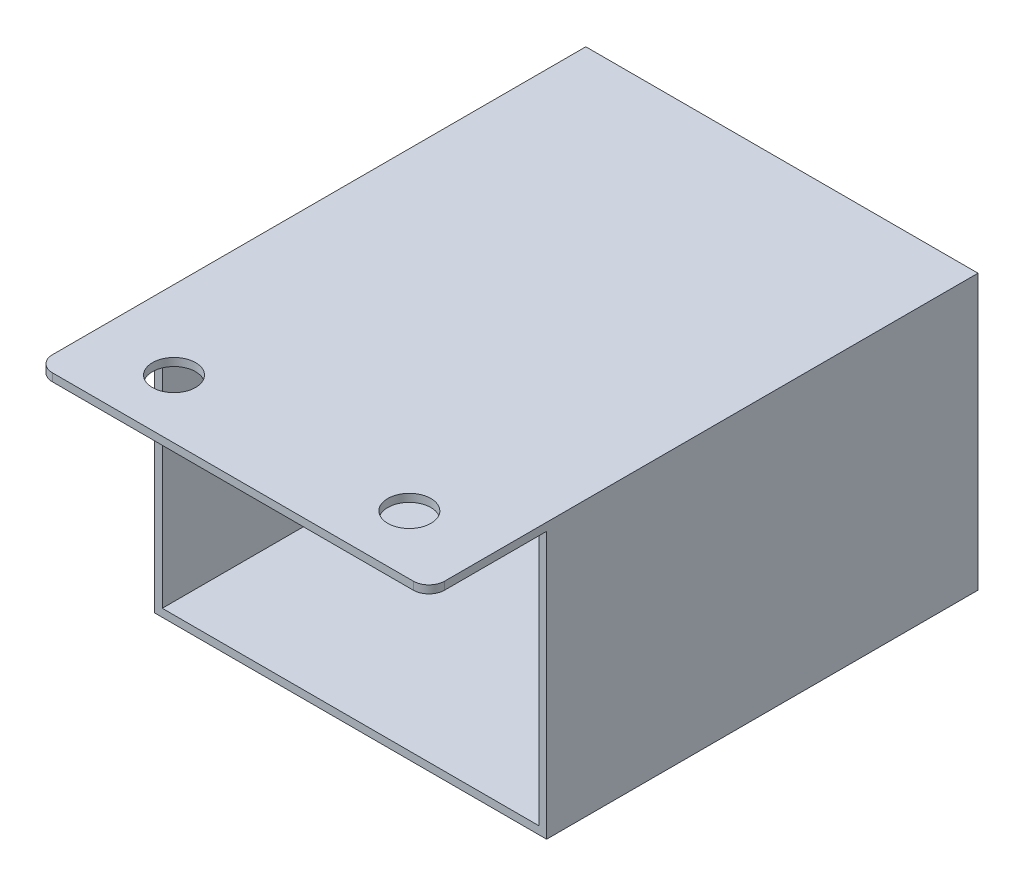
SolidWorks part; units mm, degrees
ref_plane "前视基准面" through (0, 0, 0) normal (0, 0, 1) x (1, 0, 0)
ref_plane "上视基准面" through (0, 0, 0) normal (0, 1, 0) x (1, 0, 0)
ref_plane "右视基准面" through (0, 0, 0) normal (1, 0, 0) x (0, 0, -1)
sketch "草图1" plane through (0, 0, 0) normal (0, 0, 1) x (1, 0, 0)
  line L1 (-25, 17.5) -> (25, 17.5)
  line L2 (-25, 17.5) -> (-25, -17.5)
  line L3 (-25, -17.5) -> (25, -17.5)
  line L4 (25, 17.5) -> (25, -17.5)
  line L5 (-25, 17.5) -> (25, -17.5) construction
  line L6 (-25, -17.5) -> (25, 17.5) construction
  point P0 (0, 0)
  dimension "D1" = 35
  dimension "D2" = 50
extrude "凸台-拉伸1" add sketch "草图1" along normal blind 55
sketch "草图2" plane through (0, 0, 55) normal (0, 0, 1) x (1, 0, 0)
  line L0 (25, 17.5) -> (-25, 17.5) construction
  line L1 (24, 16.5) -> (-24, 16.5)
  line L2 (24, 16.5) -> (24, -16.5)
  line L3 (24, -16.5) -> (-24, -16.5)
  line L4 (-24, 16.5) -> (-24, -16.5)
  line L5 (24, 16.5) -> (-24, -16.5) construction
  line L6 (24, -16.5) -> (-24, 16.5) construction
  line L7 (-25, 17.5) -> (-25, -17.5) construction
  point P0 (0, 0)
  dimension "D1" = 1
  dimension "D2" = 1
extrude "切除-拉伸1" cut sketch "草图2" against normal blind 54
sketch "草图5" plane through (0, 0, 55) normal (0, 0, 1) x (1, 0, 0)
  line L0 (25, -17.5) -> (25, 17.5) construction
  line L1 (-25, 17.5) -> (25, 17.5)
  line L2 (-25, 17.5) -> (-25, 16.5)
  line L3 (-25, 16.5) -> (25, 16.5)
  line L4 (25, 17.5) -> (25, 16.5)
extrude "凸台-拉伸2" add sketch "草图5" along normal blind 15
sketch "草图6" plane through (0, 16.5, 0) normal (0, -1, 0) x (1, 0, 0)
  line L0 (-25, 70) -> (-25, 55) construction
  line L1 (25, 70) -> (25, 55) construction
  line L2 (-25, 70) -> (25, 70) construction
  circle A0 centre (-15, 62.5) radius 2.75
  circle A1 centre (15, 62.5) radius 2.75
  dimension "D1" = 5.5
  dimension "D2" = 5.5
  dimension "D3" = 10
  dimension "D4" = 10
  dimension "D5" = 7.5
  dimension "D6" = 7.5
extrude "切除-拉伸3" cut sketch "草图6" against normal blind 12
fillet "圆角1" radius 2 2 edges at (25, 17, 70) (-25, 17, 70)
